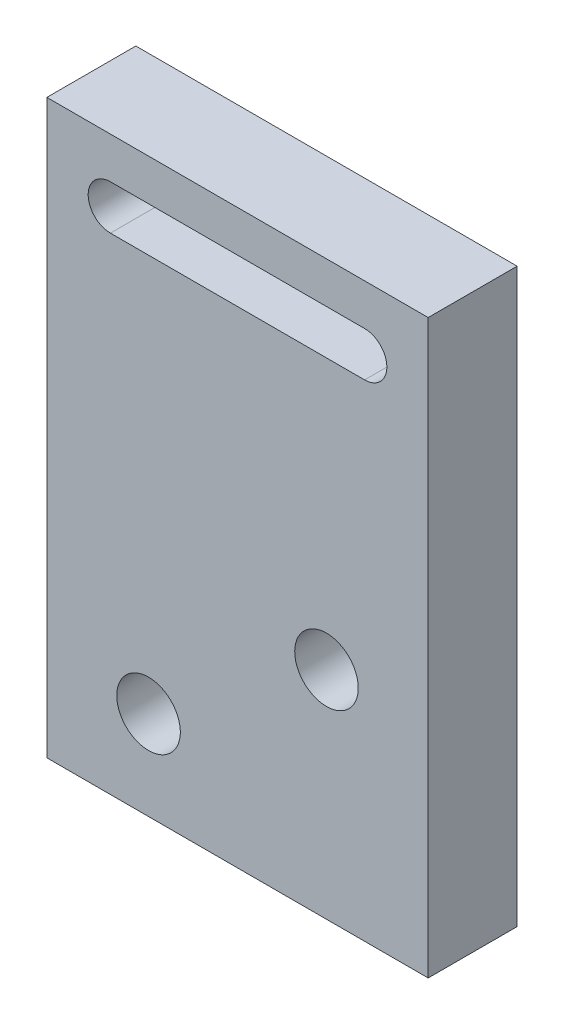
from build123d import *

# Parameters (mm, degrees)
SKETCH_1_W           = 30
SKETCH_1_H           = 45
BOSS_EXTRUDE_1_DEPTH = 7
CUT_EXTRUDE_1_DEPTH  = 28.932955447
M6_TAPPED_HOLE_1_D   = 5


with BuildPart() as part:
    # Sketch 1 → Boss-Extrude 1 (new body)
    with BuildSketch(Plane.XY):
        Rectangle(SKETCH_1_W, SKETCH_1_H)
    extrude(amount=BOSS_EXTRUDE_1_DEPTH)

    # Sketch 2 → Cut-Extrude 1 (cut, through all)
    with BuildSketch(Plane(origin=(0, 0, 0), x_dir=(-1, 0, 0), z_dir=(0, 0, -1))):
        with BuildLine():
            Line((10, 15.75), (-10, 15.75))
            ThreePointArc((-10, 15.75), (-11.75, 17.5), (-10, 19.25))
            Line((-10, 19.25), (10, 19.25))
            ThreePointArc((10, 19.25), (11.75, 17.5), (10, 15.75))
        make_face()
    extrude(amount=-CUT_EXTRUDE_1_DEPTH, mode=Mode.SUBTRACT)

    # M6 Tapped Hole 1 (through all)
    with Locations(Plane(origin=(0, 0, 0), x_dir=(-1, 0, 0), z_dir=(0, 0, -1))):
        with Locations((7, -15.5), (-7, -5.5)):
            Hole(M6_TAPPED_HOLE_1_D / 2)


solid = part.part
